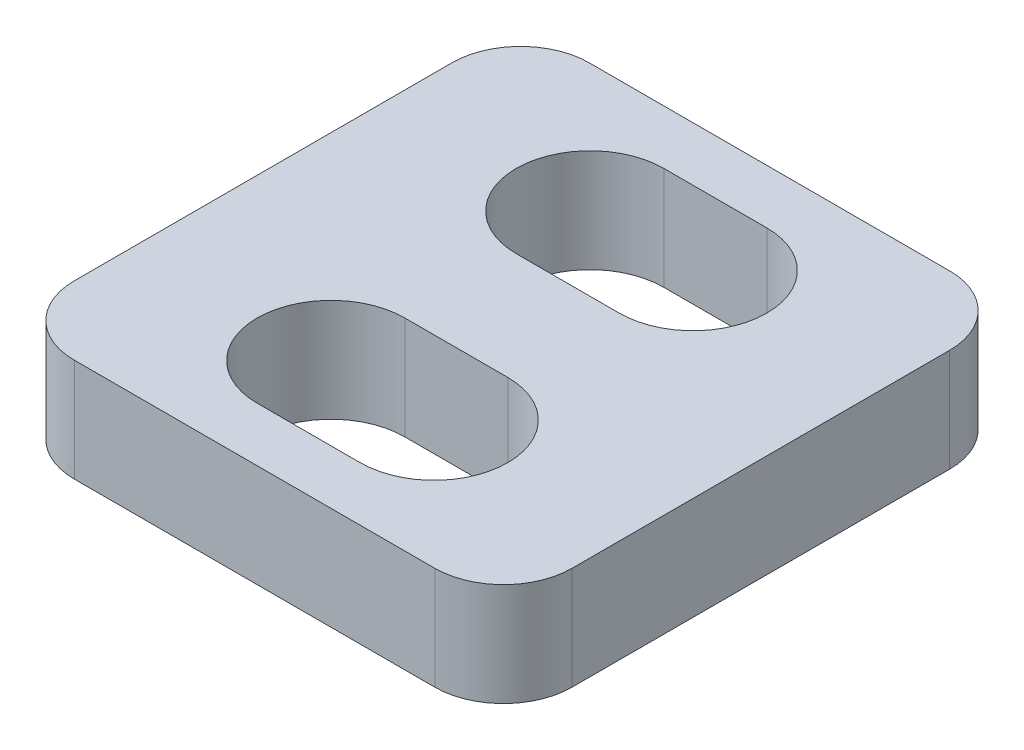
SolidWorks part; units mm, degrees
material "不锈钢201"
ref_plane "前视基准面" through (0, 0, 0) normal (0, 0, 1) x (1, 0, 0)
ref_plane "上视基准面" through (0, 0, 0) normal (0, 1, 0) x (1, 0, 0)
ref_plane "右视基准面" through (0, 0, 0) normal (1, 0, 0) x (0, 0, -1)
sketch "草图1" plane through (0, 0, 0) normal (0, 1, 0) x (1, 0, 0)
  line L1 (-7.25, 7.5) -> (7.25, 7.5)
  line L2 (-7.25, 7.5) -> (-7.25, -7.5)
  line L3 (-7.25, -7.5) -> (7.25, -7.5)
  line L4 (7.25, 7.5) -> (7.25, -7.5)
  line L5 (-7.25, 7.5) -> (7.25, -7.5) construction
  line L6 (-7.25, -7.5) -> (7.25, 7.5) construction
  point P0 (0, 0)
  dimension "D1" = 15
  dimension "D2" = 14.5
extrude "凸台-拉伸1" add sketch "草图1" along normal blind 3
sketch "草图4" plane through (0, 0, 0) normal (0, -1, 0) x (1, 0, 0)
  line L0 (1.5, -3.7725) -> (-1.5, -3.7725) construction
  line L1 (1.5, -5.9225) -> (-1.5, -5.9225)
  line L2 (1.5, -1.6225) -> (-1.5, -1.6225)
  line L3 (0, 0) -> (-10.5839, 0) construction
  line L4 (1.5, 3.7725) -> (-1.5, 3.7725) construction
  line L5 (1.5, 5.9225) -> (-1.5, 5.9225)
  line L6 (1.5, 1.6225) -> (-1.5, 1.6225)
  arc A0 (1.5, -5.9225) -> (1.5, -1.6225) centre (1.5, -3.7725) ccw
  arc A1 (-1.5, -1.6225) -> (-1.5, -5.9225) centre (-1.5, -3.7725) ccw
  arc A2 (1.5, 5.9225) -> (1.5, 1.6225) centre (1.5, 3.7725) cw
  arc A3 (-1.5, 1.6225) -> (-1.5, 5.9225) centre (-1.5, 3.7725) cw
  point P2 (0, -3.7725)
  point P12 (0, 3.7725)
  dimension "D2" = 2.15
  dimension "D1" = 3
extrude "切除-拉伸1" cut sketch "草图4" against normal blind 10
fillet "圆角1" radius 2 4 edges at (7.25, 1.5, -7.5) (-7.25, 1.5, -7.5) (-7.25, 1.5, 7.5) (7.25, 1.5, 7.5)
